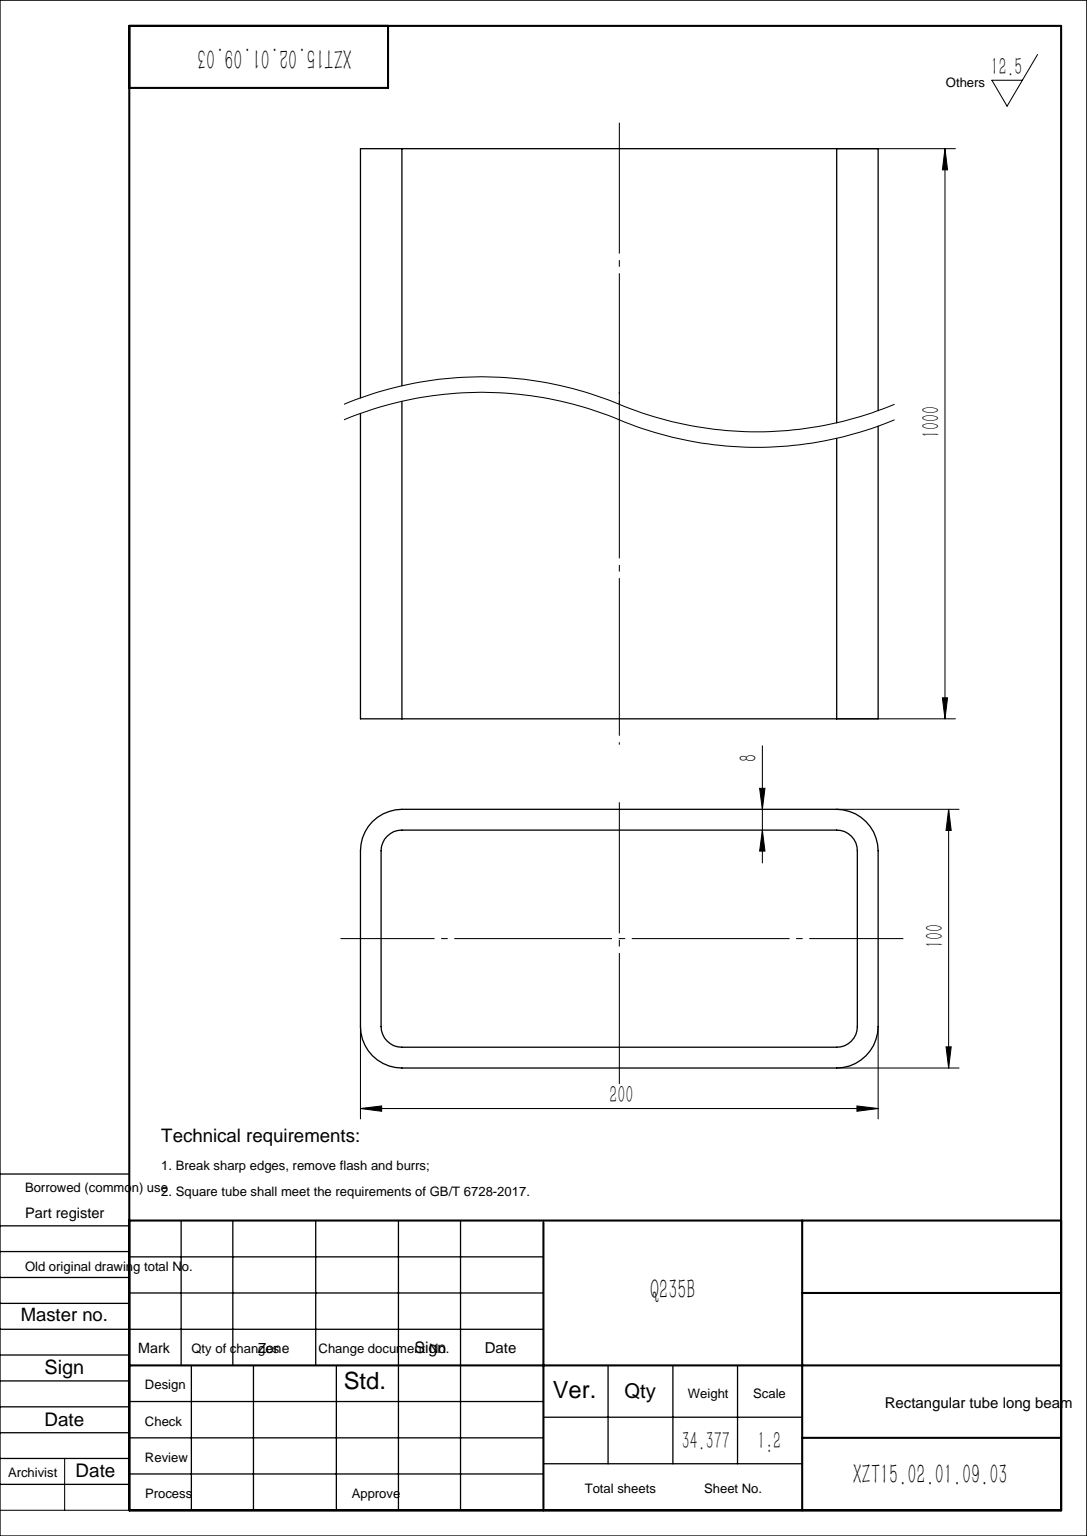
from build123d import *

# Parameters (mm, degrees)
GB_T_6728_2002_RECTANGULAR_HOLLOW_SECTIO_DEPTH = 1000


with BuildPart() as part:
    # Sketch12 → GB/T 6728-2002 rectangular hollow section 200X100X8(2) (new body)
    with BuildSketch(Plane.ZX):
        with BuildLine():
            Line((-34, -100), (34, -100))
            ThreePointArc((34, -100), (45.313708499, -95.313708499), (50, -84))
            Line((50, -84), (50, 84))
            ThreePointArc((50, 84), (45.313708499, 95.313708499), (34, 100))
            Line((34, 100), (-34, 100))
            ThreePointArc((-34, 100), (-45.313708499, 95.313708499), (-50, 84))
            Line((-50, 84), (-50, -84))
            ThreePointArc((-50, -84), (-45.313708499, -95.313708499), (-34, -100))
        make_face()
        with BuildLine():
            Line((-34, -92), (34, -92))
            ThreePointArc((34, -92), (39.656854249, -89.656854249), (42, -84))
            Line((42, -84), (42, 84))
            ThreePointArc((42, 84), (39.656854249, 89.656854249), (34, 92))
            Line((34, 92), (-34, 92))
            ThreePointArc((-34, 92), (-39.656854249, 89.656854249), (-42, 84))
            Line((-42, 84), (-42, -84))
            ThreePointArc((-42, -84), (-39.656854249, -89.656854249), (-34, -92))
        make_face(mode=Mode.SUBTRACT)
    extrude(amount=GB_T_6728_2002_RECTANGULAR_HOLLOW_SECTIO_DEPTH)


solid = part.part
